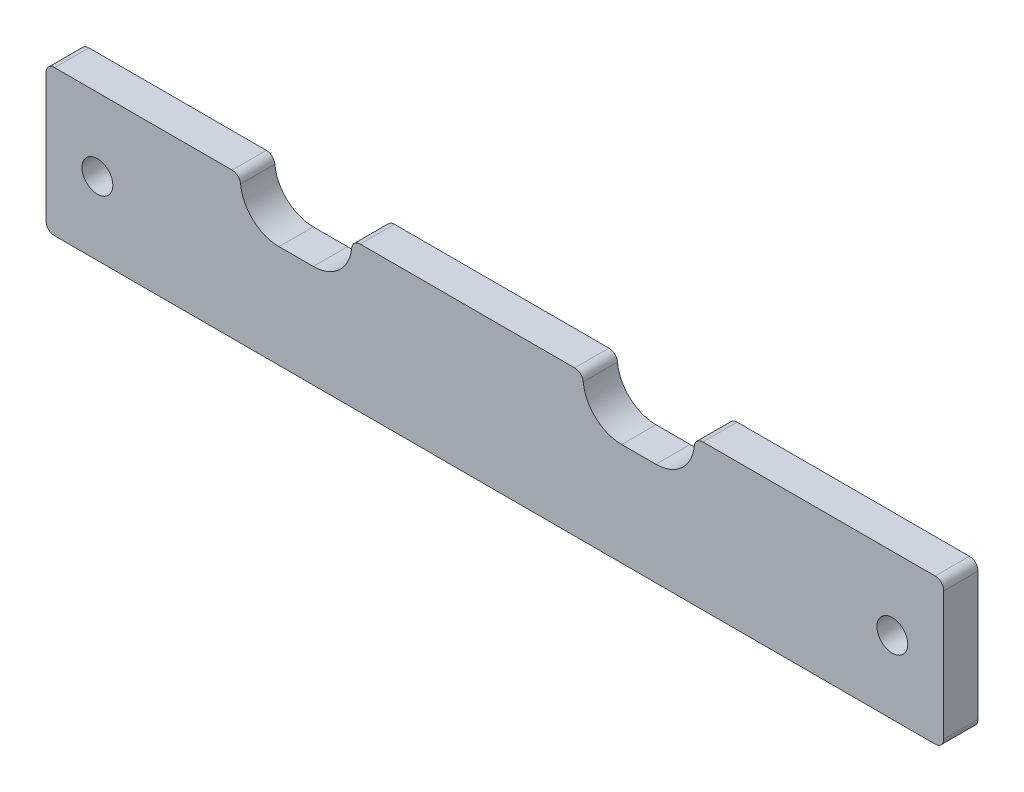
from build123d import *

# Parameters (mm, degrees)
SKETCH1_R           = 9
BOSS_EXTRUDE1_DEPTH = 20


with BuildPart() as part:
    # Sketch1 → Boss-Extrude1 (new body)
    with BuildSketch(Plane.XY):
        with BuildLine():
            Line((-26685.045416981, 9467.963220498), (-26685.045416981, 9542.963223042))
            ThreePointArc((-26685.045416981, 9542.963223042), (-26683.580949969, 9546.498755277), (-26680.045416963, 9547.96322043))
            Line((-26680.045416963, 9547.96322043), (-26576.431543676, 9547.96322043))
            ThreePointArc((-26576.431543676, 9547.96322043), (-26573.060544526, 9546.655965332), (-26571.452248862, 9543.417765798))
            ThreePointArc((-26571.452248862, 9543.417765798), (-26564.214913831, 9528.845869116), (-26549.045416948, 9522.963220428))
            Line((-26549.045416948, 9522.963220428), (-26529.045416963, 9522.963220428))
            ThreePointArc((-26529.045416963, 9522.963220428), (-26513.875918272, 9528.845870766), (-26506.638584632, 9543.417770687))
            ThreePointArc((-26506.638584632, 9543.417770687), (-26505.030289423, 9546.655967321), (-26501.659292496, 9547.963220408))
            Line((-26501.659292496, 9547.963220408), (-26376.431544058, 9547.963220408))
            ThreePointArc((-26376.431544058, 9547.963220408), (-26373.060544852, 9546.655965256), (-26371.452248862, 9543.417765804))
            ThreePointArc((-26371.452248862, 9543.417765804), (-26364.214913847, 9528.845869098), (-26349.045416954, 9522.963220397))
            Line((-26349.045416954, 9522.963220397), (-26329.045416961, 9522.963220397))
            ThreePointArc((-26329.045416961, 9522.963220397), (-26313.875920919, 9528.845868323), (-26306.638585232, 9543.417763496))
            ThreePointArc((-26306.638585232, 9543.417763496), (-26305.03028784, 9546.655964088), (-26301.659287339, 9547.963220451))
            Line((-26301.659287339, 9547.963220451), (-26289.045416951, 9547.963220451))
            Line((-26289.045416951, 9547.963220451), (-26166.045416928, 9547.963220451))
            ThreePointArc((-26166.045416928, 9547.963220451), (-26162.509883026, 9546.498754363), (-26161.045416939, 9542.96322046))
            Line((-26161.045416939, 9542.96322046), (-26161.045416939, 9467.96322112))
            ThreePointArc((-26161.045416939, 9467.96322112), (-26162.509882821, 9464.42768677), (-26166.045416981, 9462.96322043))
            Line((-26166.045416981, 9462.96322043), (-26680.045417049, 9462.96322043))
            ThreePointArc((-26680.045417049, 9462.96322043), (-26683.580950913, 9464.427686595), (-26685.045416981, 9467.963220498))
        make_face()
        with Locations((-26655.045416981, 9505.46322043)):
            Circle(SKETCH1_R, mode=Mode.SUBTRACT)
        with Locations((-26191.045416981, 9505.46322043)):
            Circle(SKETCH1_R, mode=Mode.SUBTRACT)
    extrude(amount=BOSS_EXTRUDE1_DEPTH)


solid = part.part
